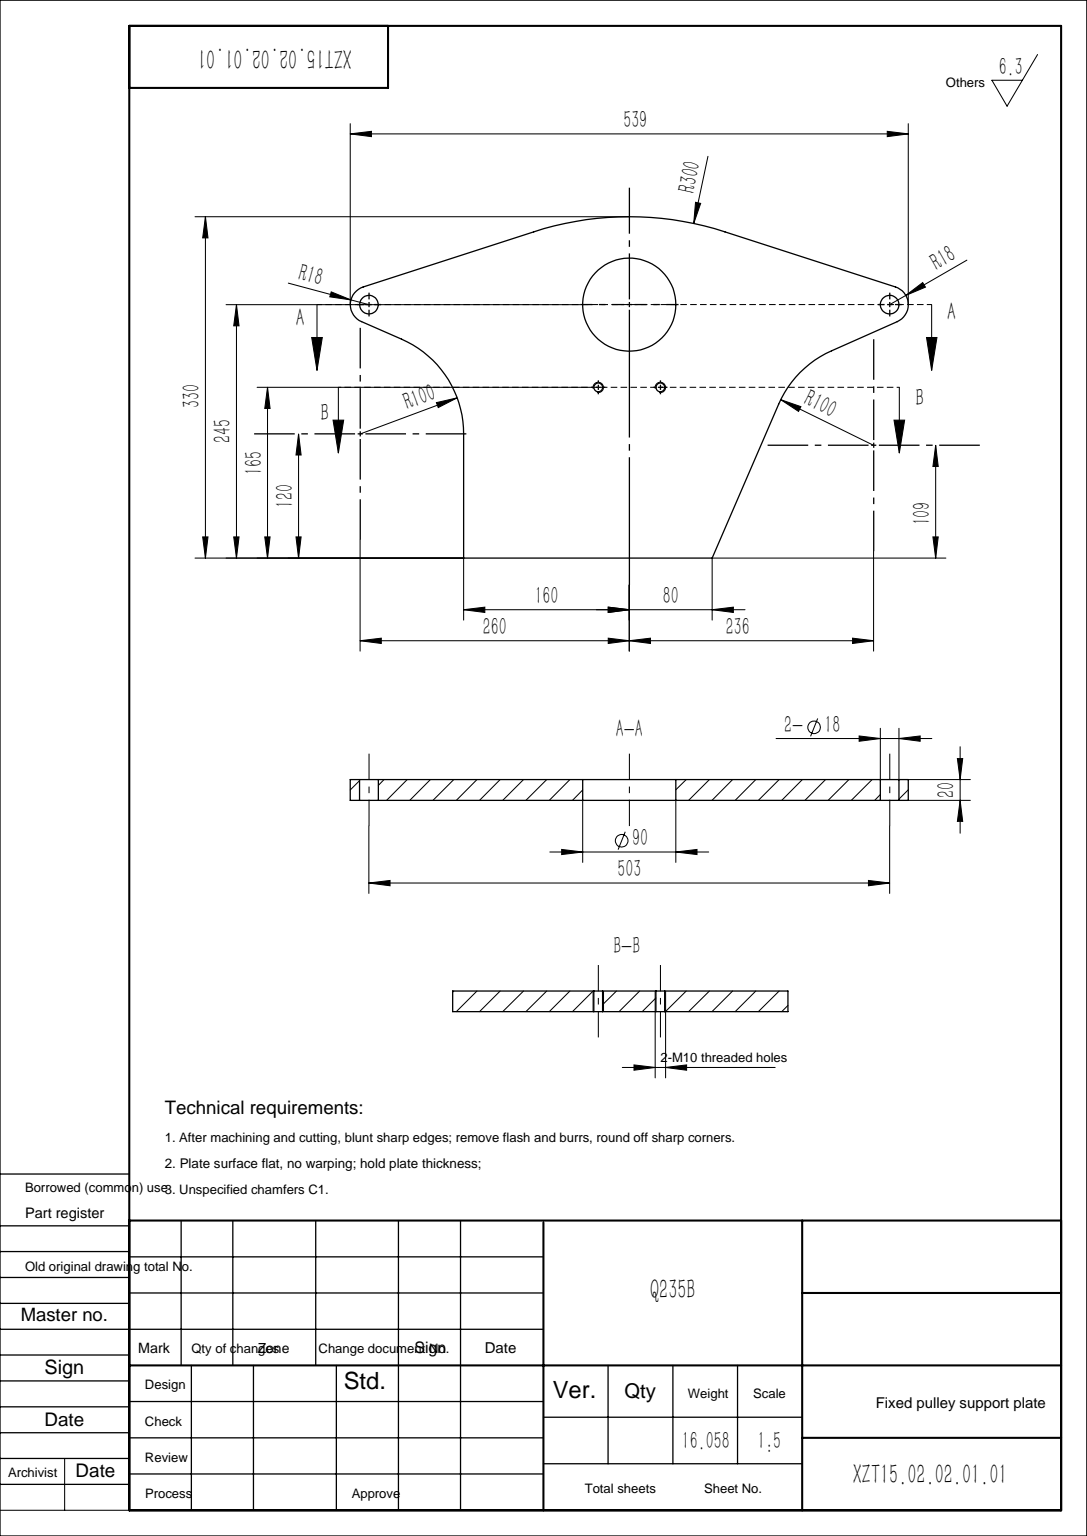
SolidWorks part; units mm, degrees
material "Q235B"
ref_plane "Front Plane" through (0, 0, 0) normal (0, 0, 1) x (1, 0, 0)
ref_plane "Top Plane" through (0, 0, 0) normal (0, 1, 0) x (1, 0, 0)
ref_plane "Right Plane" through (0, 0, 0) normal (1, 0, 0) x (0, 0, -1)
sketch "Sketch1" plane through (0, 0, 0) normal (0, 0, 1) x (1, 0, 0)
  line L0 (0, 0) -> (-160, 0)
  line L1 (-160, 0) -> (-160, 120)
  line L2 (-257.043, 262.1253) -> (-92.3834, 315.4213)
  line L3 (0, 0) -> (80, 0)
  line L4 (80, 0) -> (144.1953, 148.6471)
  line L6 (257.043, 262.1253) -> (92.3834, 315.4213)
  line L7 (-220.0774, 211.6853) -> (-258.6861, 228.4967)
  line L8 (195.4082, 200.391) -> (258.8065, 228.5496)
  line L9 (0, 0) -> (0, 245) construction
  arc A0 (-160, 120) -> (-220.0774, 211.6853) centre (-260, 120) ccw
  arc A2 (-92.3834, 315.4213) -> (92.3834, 315.4213) centre (0, 30) cw
  arc A3 (144.1953, 148.6471) -> (195.4082, 200.391) centre (236, 109) cw
  arc A4 (258.8065, 228.5496) -> (257.043, 262.1253) centre (251.5, 245) ccw
  arc A5 (-258.6861, 228.4967) -> (-257.043, 262.1253) centre (-251.5, 245) cw
  circle A6 centre (0, 245) radius 45
  circle A7 centre (-251.5, 245) radius 9
  circle A8 centre (251.5, 245) radius 9
  dimension "D1" = 160
  dimension "D3" = 100
  dimension "D4" = 100
  dimension "D5" = 18
  dimension "D6" = 300
  dimension "D7" = 18
  dimension "D8" = 539
  dimension "D9" = 330
  dimension "D11" = 90
  dimension "D12" = 18
  dimension "D13" = 18
  dimension "D2" = 80
  dimension "D10" = 245
  dimension "D14" = 120
  dimension "D15" = 109
  dimension "D16" = 236
extrude "Boss-Extrude1" add sketch "Sketch1" along normal mid plane 20
hole_wizard "M10 Tapped Hole1" positions "Sketch2" profile "Sketch3" tap size "M10" standard "GB" end condition up to next
sketch "Sketch2" plane through (0, 0, 10) normal (0, 0, 1) x (1, 0, 0)
  line L0 (0, 0) -> (0, 157.1161) construction
  line L2 (-160, 0) -> (80, 0) construction
  point P0 (-30, 165)
  point P7 (30, 165)
  dimension "D1" = 165
  dimension "D2" = 60
sketch "Sketch3" plane through (-30, 165, 10) normal (1, 0, 0) x (0, -1, 0)
  line L0 (0, 0) -> (0, 20)
  line L1 (0, 20) -> (4.25, 20)
  line L2 (4.25, 20) -> (4.25, 0)
  line L5 (4.25, 0) -> (0, 0)
  line L11 (0, -6.35) -> (0, 107.95) construction
  dimension "通孔螺纹孔钻头直径" = 8.5
  dimension "通孔螺纹孔钻头深度" = 20
cosmetic thread "Cosmetic thread1" parameters "D2"=10
cosmetic thread "Cosmetic thread2" parameters "D2"=10
